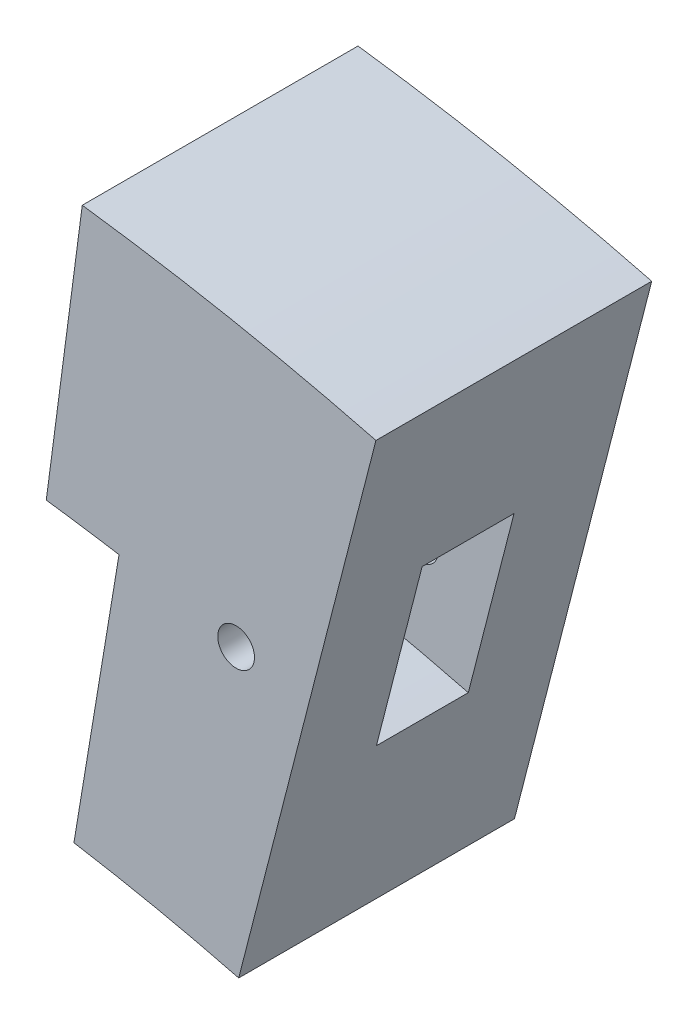
SolidWorks part; units mm, degrees
ref_plane "Front Plane" through (0, 0, 0) normal (0, 0, 1) x (1, 0, 0)
ref_plane "Top Plane" through (0, 0, 0) normal (0, 1, 0) x (1, 0, 0)
ref_plane "Right Plane" through (0, 0, 0) normal (1, 0, 0) x (0, 0, -1)
sketch "Sketch1" plane through (0, 0, 0) normal (0, 0, 1) x (1, 0, 0)
  line L1 (6.9641, 114.7889) -> (9.1888, 134.6869)
  line L2 (17.1673, 103.5871) -> (18.8023, 113.4525)
  line L3 (26.1302, 101.6967) -> (33.596, 130.7529)
  arc A0 (33.596, 130.7529) -> (9.1888, 134.6869) centre (0, 0) ccw
  arc A1 (26.1302, 101.6967) -> (17.1673, 103.5871) centre (0, 0) ccw
  arc A3 (18.8023, 113.4525) -> (6.9641, 114.7889) centre (0, 0) ccw
  dimension "D1" = 270
  dimension "D2" = 210
  dimension "D5" = 230
  dimension "D7" = 5
extrude "Boss-Extrude1" add sketch "Sketch1" along normal blind 15
sketch "Sketch3" plane through (0, 0, 15) normal (0, 0, 1) x (1, 0, 0)
  line L0 (28.6188, 111.3821) -> (31.1074, 121.0675)
  line L1 (26.1302, 101.6967) -> (33.596, 130.7529) construction
  line L2 (8.0764, 124.7379) -> (6.9641, 114.7889)
  line L3 (9.1888, 134.6869) -> (6.9641, 114.7889) construction
  arc A1 (28.6188, 111.3821) -> (6.9641, 114.7889) centre (0, 0) ccw
  arc A2 (8.0764, 124.7379) -> (31.1071, 121.0666) centre (0, 0) cw
  line M4 (9.1888, 134.6869) -> (6.9641, 114.7889)
  arc M5 (6.9641, 114.7889) -> (18.8023, 113.4525) centre (0, 0) cw
  line M8 (26.1302, 101.6967) -> (33.596, 130.7529)
  dimension "D1" = 125
extrude "Cut-Extrude1" cut sketch "Sketch3" against normal blind 10 contours A2 A1 M4 M5 M8
sketch "Sketch4" plane through (0, 0, 15) normal (0, 0, 1) x (1, 0, 0)
  line L0 (0, 0) -> (0.0973, 0.3786)
  line L1 (0, -1.2422) -> (0.0973, 0.3786)
  line L2 (6.9641, 114.7889) -> (8.0764, 124.7379)
  line L3 (28.6188, 111.3821) -> (31.1071, 121.0666)
  arc A0 (31.1071, 121.0666) -> (8.0764, 124.7379) centre (0, 0) ccw
  arc A1 (28.6188, 111.3821) -> (6.9641, 114.7889) centre (0, 0) ccw
  arc M2 (8.0764, 124.7379) -> (31.1071, 121.0666) centre (0, 0) cw
extrude "Boss-Extrude3" add sketch "Sketch4" against normal blind 5 contours A1 L3 L2 M2
sketch "Sketch5" plane through (0, 0, 15) normal (0, 0, 1) x (1, 0, 0)
  circle A0 centre (25.9889, 117.2202) radius 1
  dimension "D2" = 2
extrude "Cut-Extrude2" cut sketch "Sketch5" against normal blind 15
sketch "Sketch7" plane through (0, 0, 15) normal (0, 0, 1) x (1, 0, 0)
  line L0 (0, 115) -> (0, 135)
  line L1 (15.0105, 114.0162) -> (17.621, 133.8451)
  arc A0 (17.621, 133.8451) -> (0, 135) centre (0, 0) ccw
  arc A1 (15.0105, 114.0162) -> (0, 115) centre (0, 0) ccw
  dimension "D1" = 135
  dimension "D2" = 7.5
extrude "Cut-Extrude4" cut sketch "Sketch7" against normal blind 15
sketch "Sketch8" plane through (0, 0, 15) normal (0, 0, 1) x (1, 0, 0)
  line L0 (15.0105, 114.0162) -> (15.6631, 118.9734)
  line L1 (15.0105, 114.0162) -> (17.621, 133.8451) construction
  line L2 (18.8023, 113.4525) -> (19.6198, 118.3852)
  arc A0 (19.6198, 118.3852) -> (15.6631, 118.9734) centre (0, 0) ccw
  arc A1 (18.8023, 113.4525) -> (15.0105, 114.0162) centre (0, 0) ccw
  dimension "D1" = 120
extrude "Cut-Extrude5" cut sketch "Sketch8" against normal blind 15
